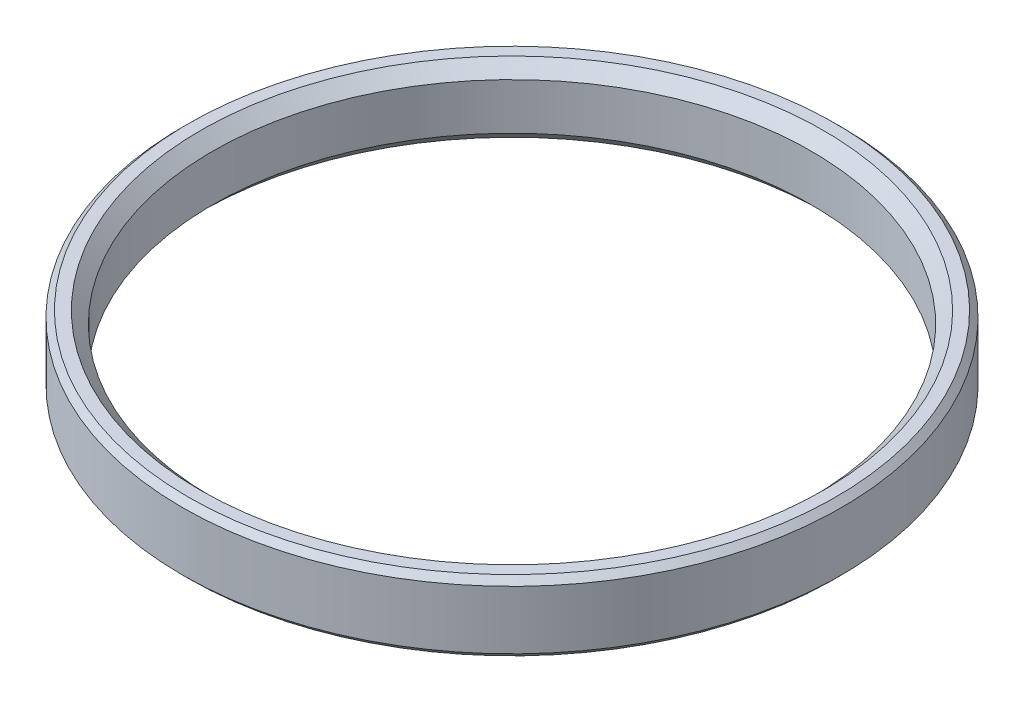
SolidWorks part; units mm, degrees
ref_plane "Front Plane" through (0, 0, 0) normal (0, 0, 1) x (1, 0, 0)
ref_plane "Top Plane" through (0, 0, 0) normal (0, 1, 0) x (1, 0, 0)
ref_plane "Right Plane" through (0, 0, 0) normal (1, 0, 0) x (0, 0, -1)
sketch "Sketch1" plane through (0, 0, 0) normal (0, 1, 0) x (1, 0, 0)
  circle A0 centre (0, 0) radius 55
  circle A1 centre (0, 0) radius 50
  dimension "D1" = 110
  dimension "D2" = 100
extrude "Boss-Extrude1" add sketch "Sketch1" along normal blind 11.75
chamfer "Chamfer1" distance 1 angle 45 2 edges at (0, 0, 55) (0, 11.75, 55)
chamfer "Chamfer2" distance 2 angle 45 2 edges at (0, 0, 50) (0, 11.75, 50)
